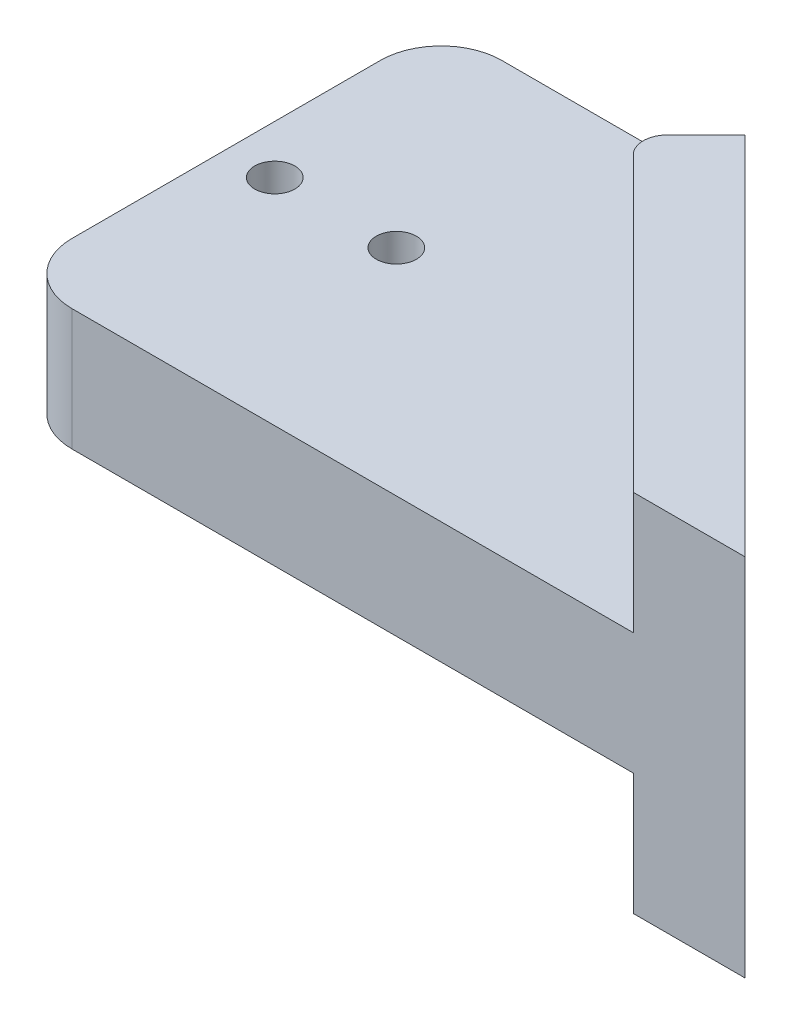
SolidWorks part; units mm, degrees
ref_plane "前视基准面" through (0, 0, 0) normal (0, 0, 1) x (1, 0, 0)
ref_plane "上视基准面" through (0, 0, 0) normal (0, 1, 0) x (1, 0, 0)
ref_plane "右视基准面" through (0, 0, 0) normal (1, 0, 0) x (0, 0, -1)
sketch "草图1" plane through (0, 0, 0) normal (0, 1, 0) x (1, 0, 0)
  line L1 (-12, -15) -> (48.3553, -15)
  line L2 (48.3553, -15) -> (13, 20.3553)
  line L3 (13, 20.3553) -> (-12, 20.3553)
  line L4 (-12, 20.3553) -> (-12, -15)
  dimension "D1" = 45
  dimension "D2" = 50
  dimension "D3" = 15
  dimension "D4" = 25
  dimension "D5" = 12
extrude "凸台-拉伸1" add sketch "草图1" along normal mid plane 10
hole_wizard "M4 螺纹孔1" positions "草图2" profile "草图3" tap size "M4" standard "ISO" end condition through all
sketch "草图2" plane through (0, -5, 0) normal (0, -1, 0) x (-1, 0, 0)
  line L0 (12, 2.6777) -> (-30.6777, 2.6777) construction
  line L1 (12, 20.3553) -> (12, -15) construction
  line L2 (-48.3553, -15) -> (-13, 20.3553) construction
  point P0 (8, 2.6777)
  point P2 (-2, 2.6777)
  dimension "D1" = 10
  dimension "D2" = 4
sketch "草图3" plane through (-8, -5, -2.6777) normal (1, 0, 0) x (0, 0, -1)
  line L0 (0, 0) -> (0, 10)
  line L1 (0, 10) -> (1.65, 10)
  line L2 (1.65, 10) -> (1.65, 0)
  line L5 (1.65, 0) -> (0, 0)
  line L11 (0, -6.35) -> (0, 107.95) construction
  dimension "通孔螺纹孔钻头直径" = 3.3
  dimension "通孔螺纹孔钻头深度" = 10
cosmetic thread "孔螺蚊线1" parameters "D2"=4
cosmetic thread "孔螺蚊线2" parameters "D2"=4
sketch "草图5" plane through (0, -5, 0) normal (0, -1, 0) x (1, 0, 0)
  line L1 (13.7071, -10.4558) -> (39.163, 15)
  line L2 (-12, 15) -> (48.3553, 15) construction
  line L3 (39.163, 15) -> (48.3553, 15)
  line L4 (48.3553, 15) -> (18.3033, -15.052)
  line L7 (18.3033, -15.052) -> (13.7071, -10.4558)
  line L9 (48.3553, 15) -> (13, -20.3553) construction
  dimension "D1" = 36
  dimension "D2" = 6.5
extrude "凸台-拉伸3" add sketch "草图5" along normal blind 10
mirror "镜向1" about plane through (0, 0, 0) normal (0, 1, 0) of "凸台-拉伸3"
hole_wizard "M4 六角凹头螺钉的柱形沉头孔1" positions "草图6" profile "草图7" counterbore size "M4" standard "ISO" end condition through all
sketch "草图6" plane through (12.0815, 0, -12.0815) normal (-0.7071, 0, 0.7071) x (0.7071, 0, 0.7071)
  circle A0 centre (30.799, 10) radius 1.65 construction
  circle A1 centre (8.799, 10) radius 1.65 construction
  circle A2 centre (8.799, -10) radius 1.65 construction
  circle A3 centre (30.799, -10) radius 1.65 construction
  point P0 (8.799, 10)
  point P2 (30.799, 10)
  point P4 (8.799, -10)
  point P6 (30.799, -10)
sketch "草图7" plane through (18.3033, 10, -5.8597) normal (0, 1, 0) x (0.7071, 0, 0.7071)
  line L0 (0, 0) -> (0, 31.5)
  line L1 (0, 31.5) -> (2.25, 31.5)
  line L3 (2.25, 31.5) -> (2.25, 4.4)
  line L4 (2.25, 4.4) -> (4, 4.4)
  line L5 (4, 4.4) -> (4, 0)
  line L7 (4, 0) -> (0, 0)
  line L11 (0, -6.35) -> (0, 107.95) construction
  dimension "通孔孔直径" = 4.5
  dimension "通孔孔深度" = 31.5
  dimension "柱形沉头孔直径" = 8
  dimension "柱形沉头孔深度" = 4.4
fillet "圆角1" radius 2 2 edges at (13.7071, 10, -10.4558) (13.7071, -10, -10.4558)
fillet "圆角2" radius 5 2 edges at (-12, 0, 15) (-12, 0, -20.3553)
